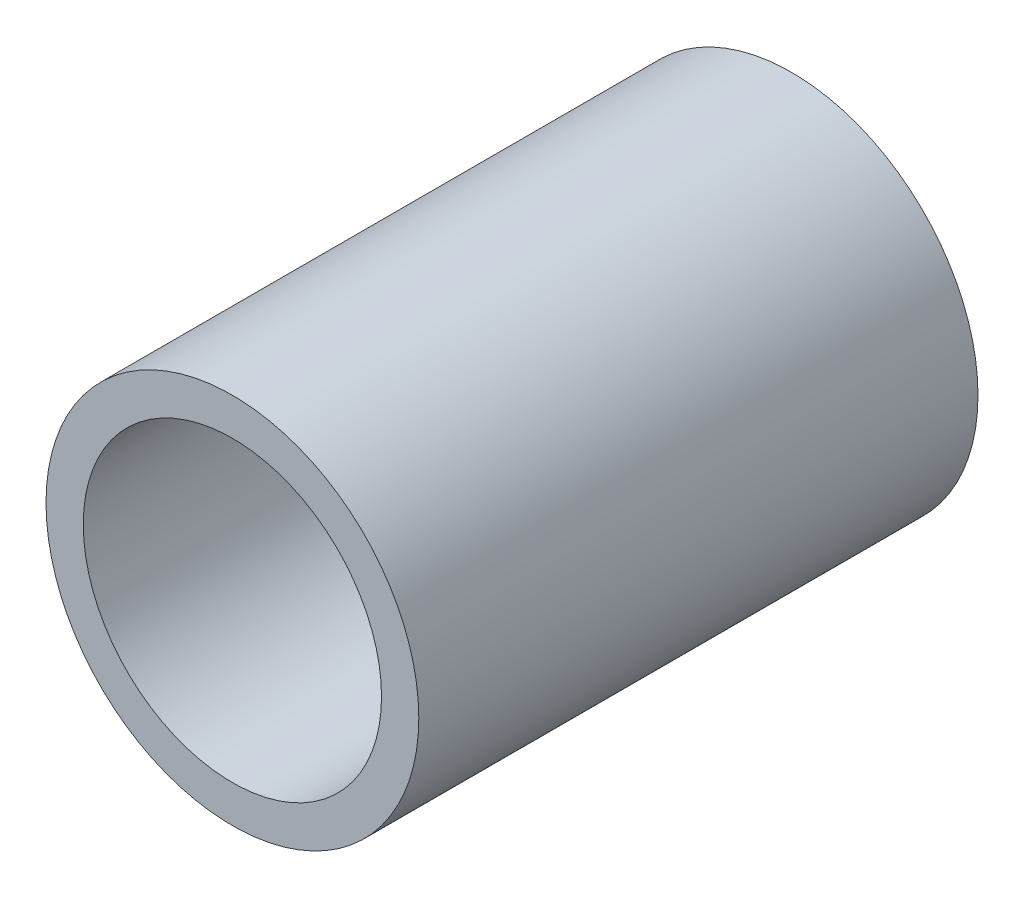
from build123d import *

# Parameters (mm, degrees)
SKETCH_1_R      = 10
SKETCH_1_R_2    = 8
EXTRUDE_1_DEPTH = 30


with BuildPart() as part:
    # 草图1 → 拉伸-薄壁1 (new body)
    with BuildSketch(Plane.XY):
        Circle(SKETCH_1_R)
        Circle(SKETCH_1_R_2, mode=Mode.SUBTRACT)
    extrude(amount=EXTRUDE_1_DEPTH)


solid = part.part
